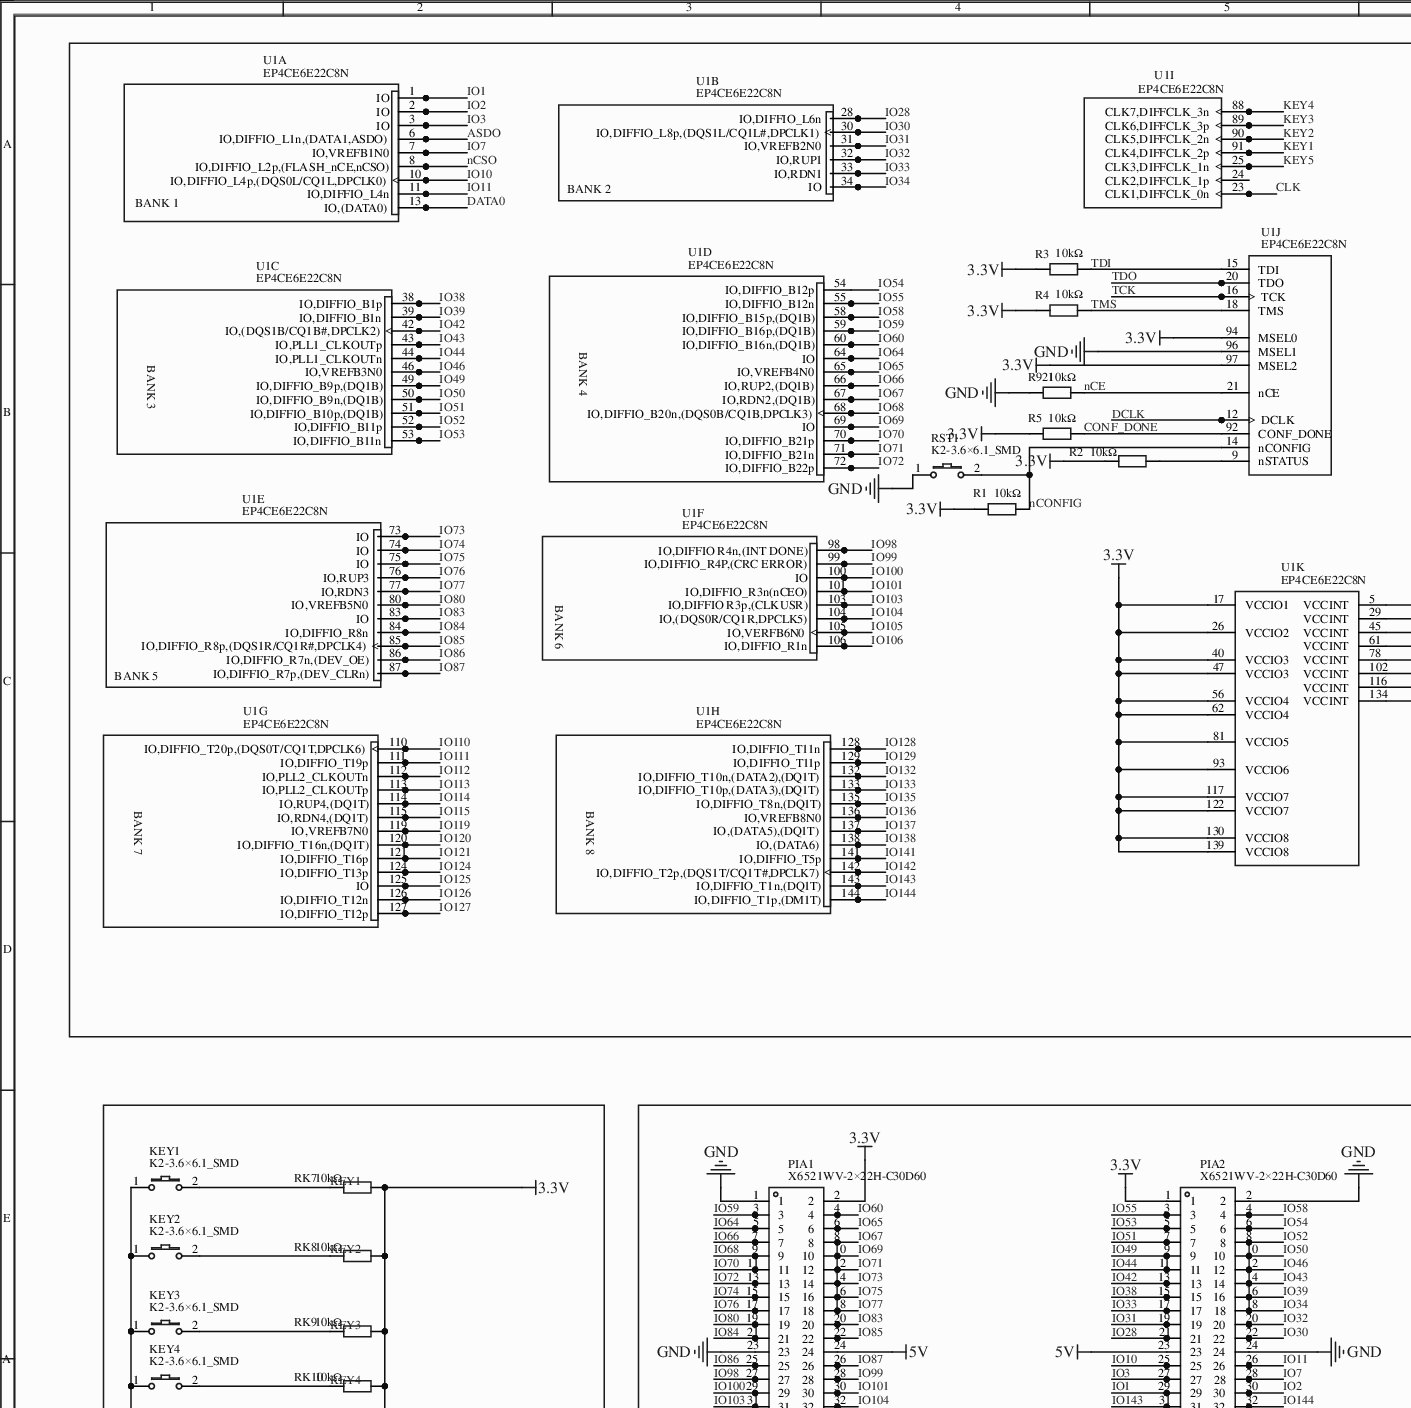
[diagram p0: MISC51540-3.schdoc, top left]
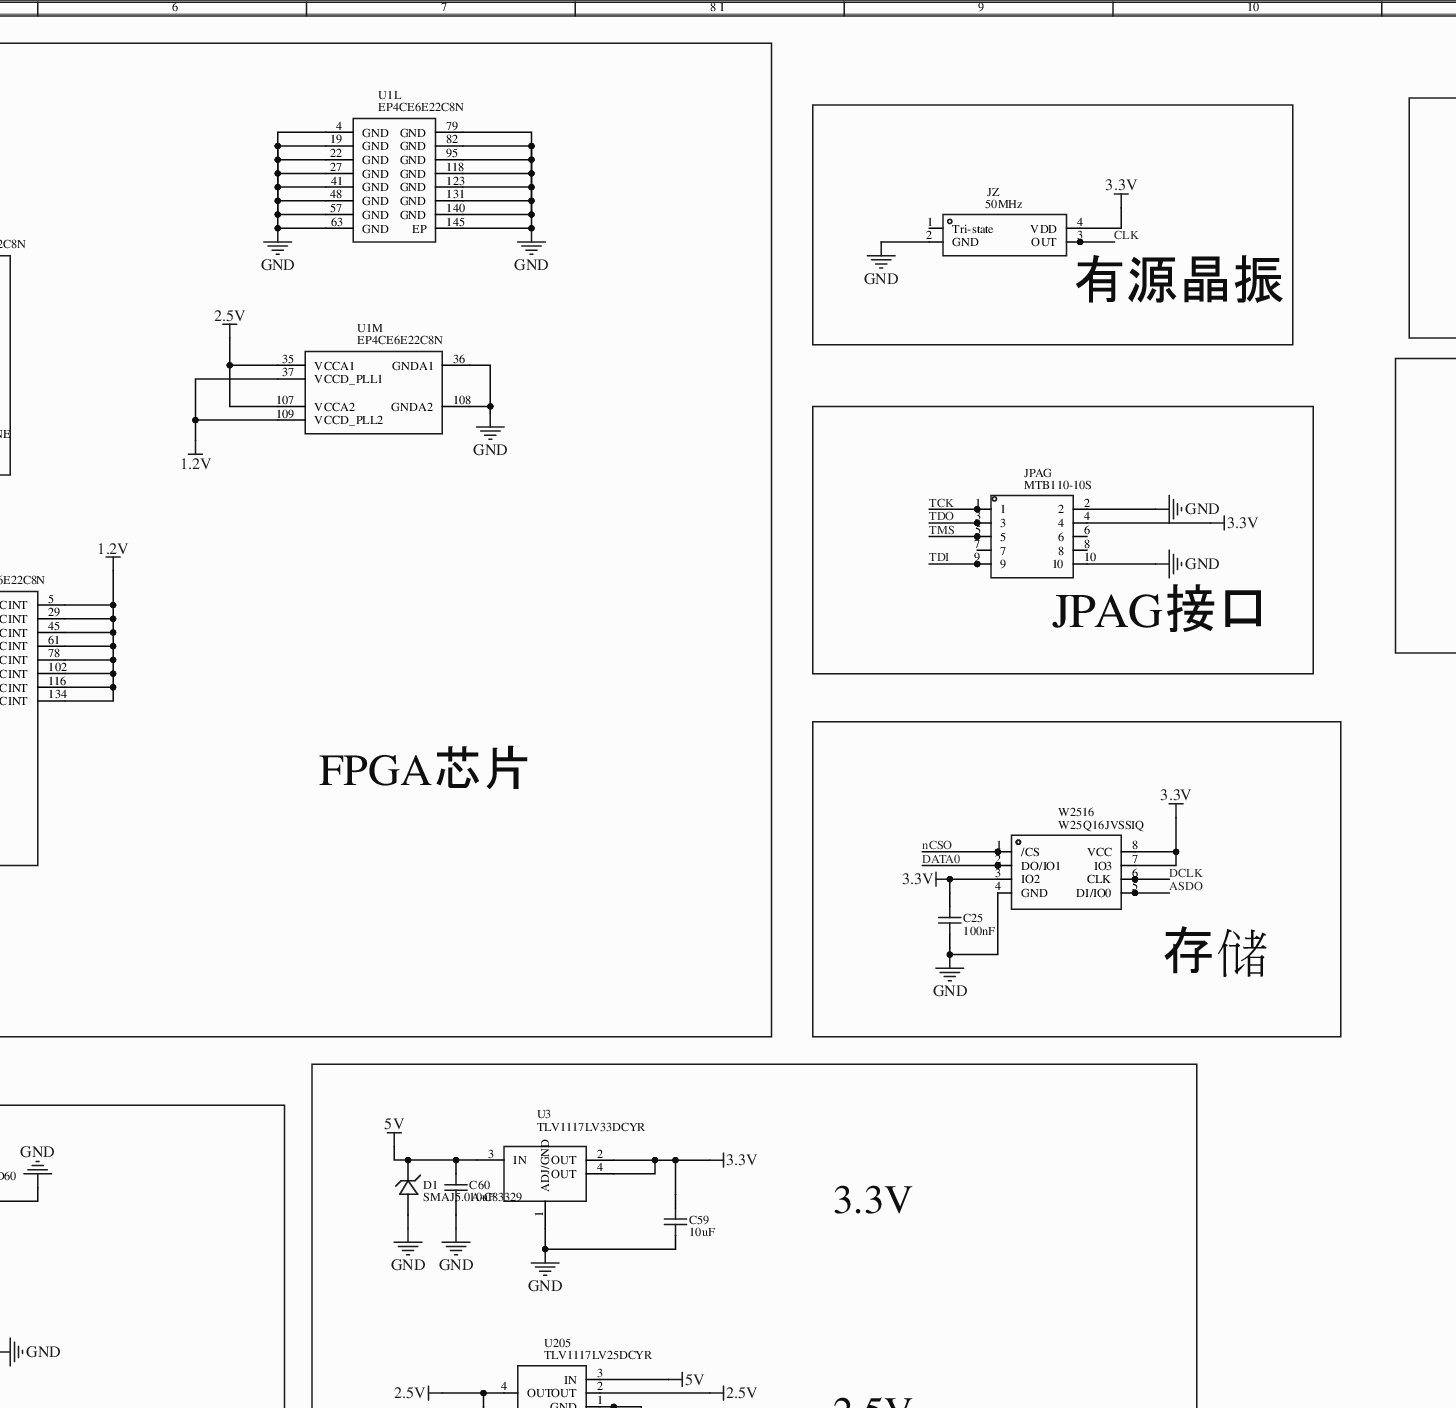
[diagram p1: MISC51540-3.schdoc, top middle]
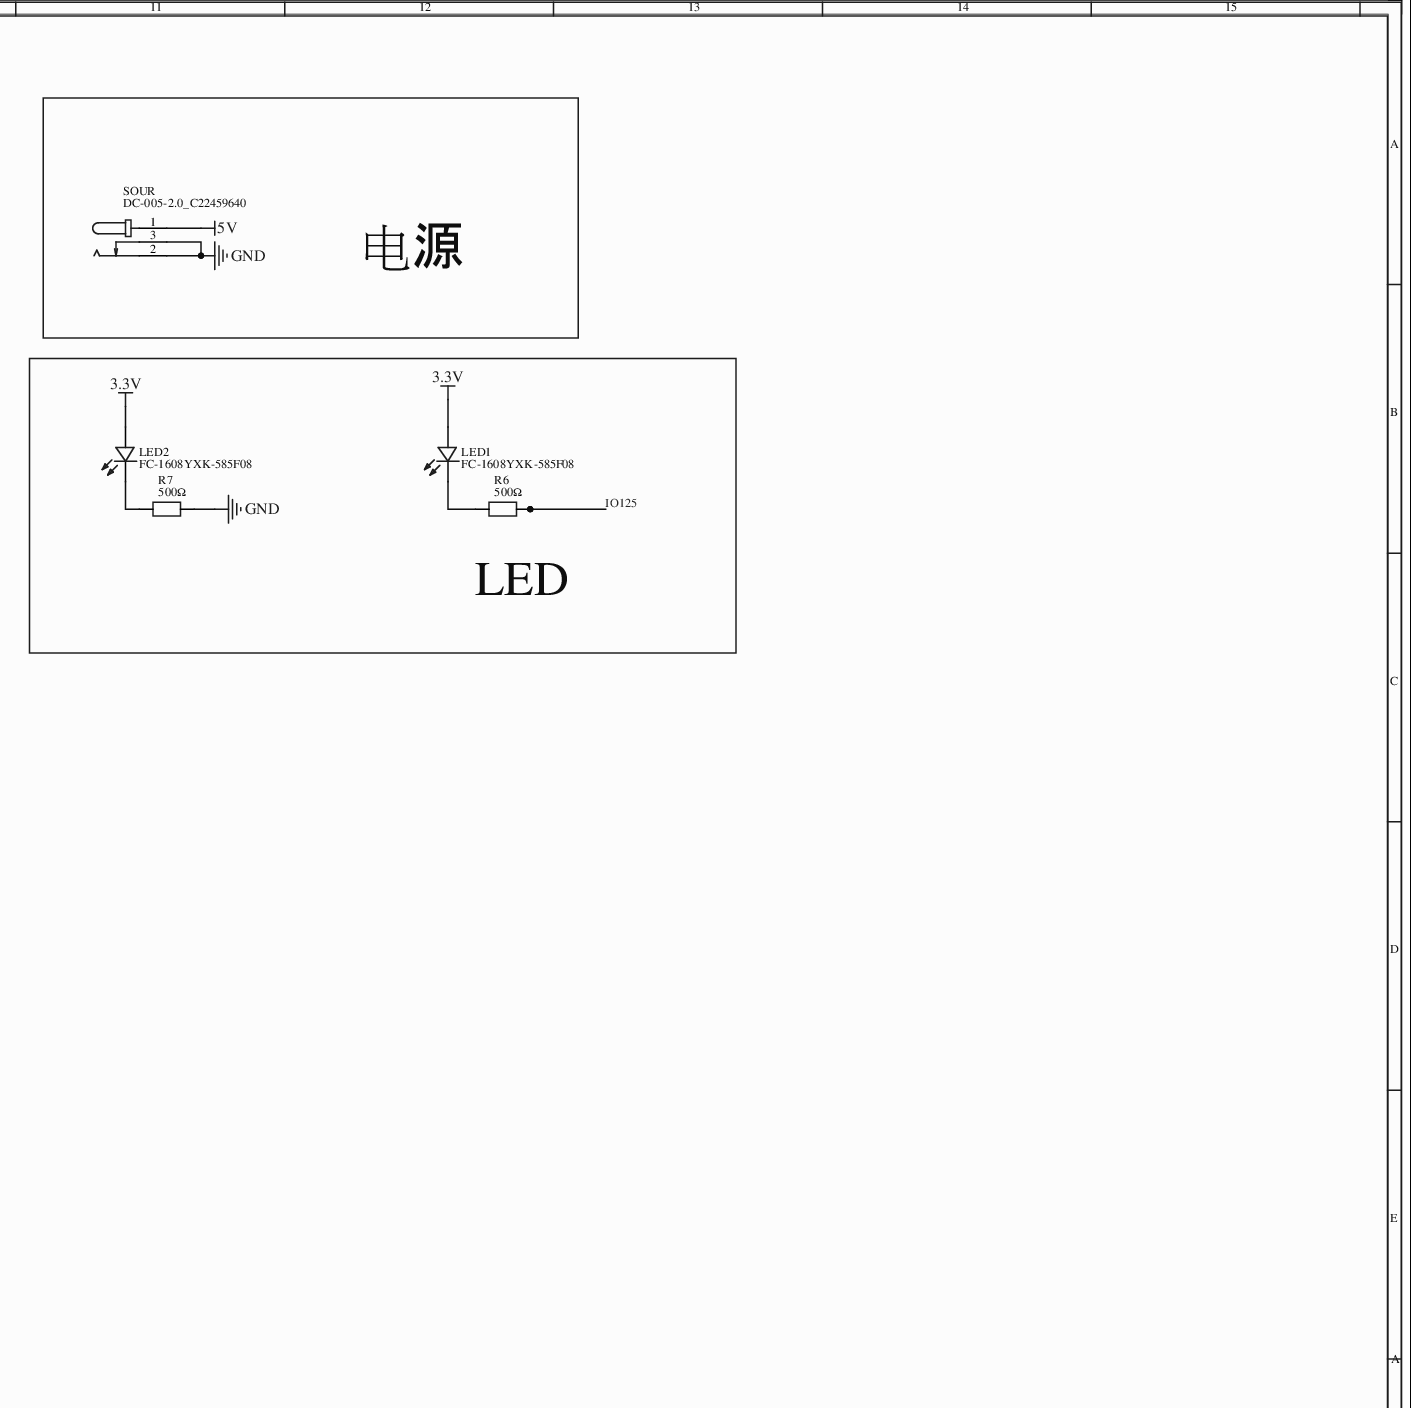
[diagram p2: MISC51540-3.schdoc, top right]
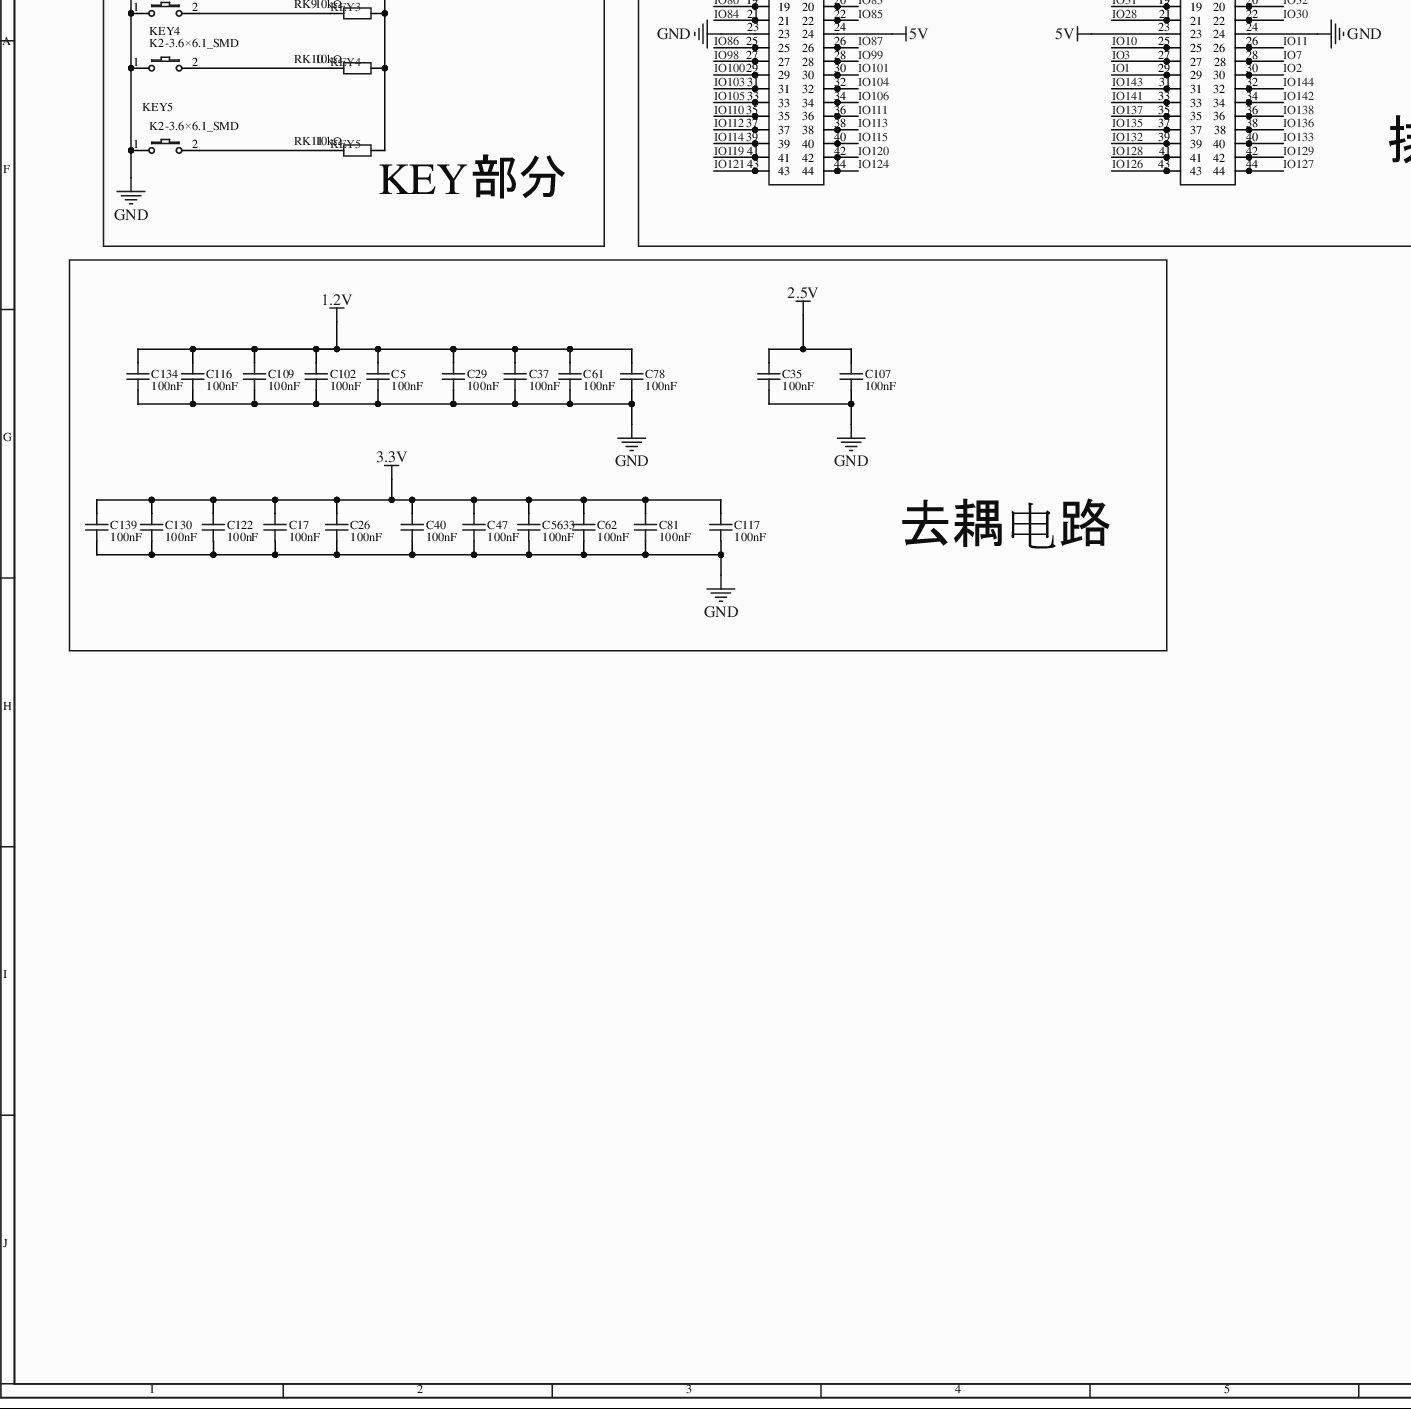
[diagram p3: MISC51540-3.schdoc, bottom left]
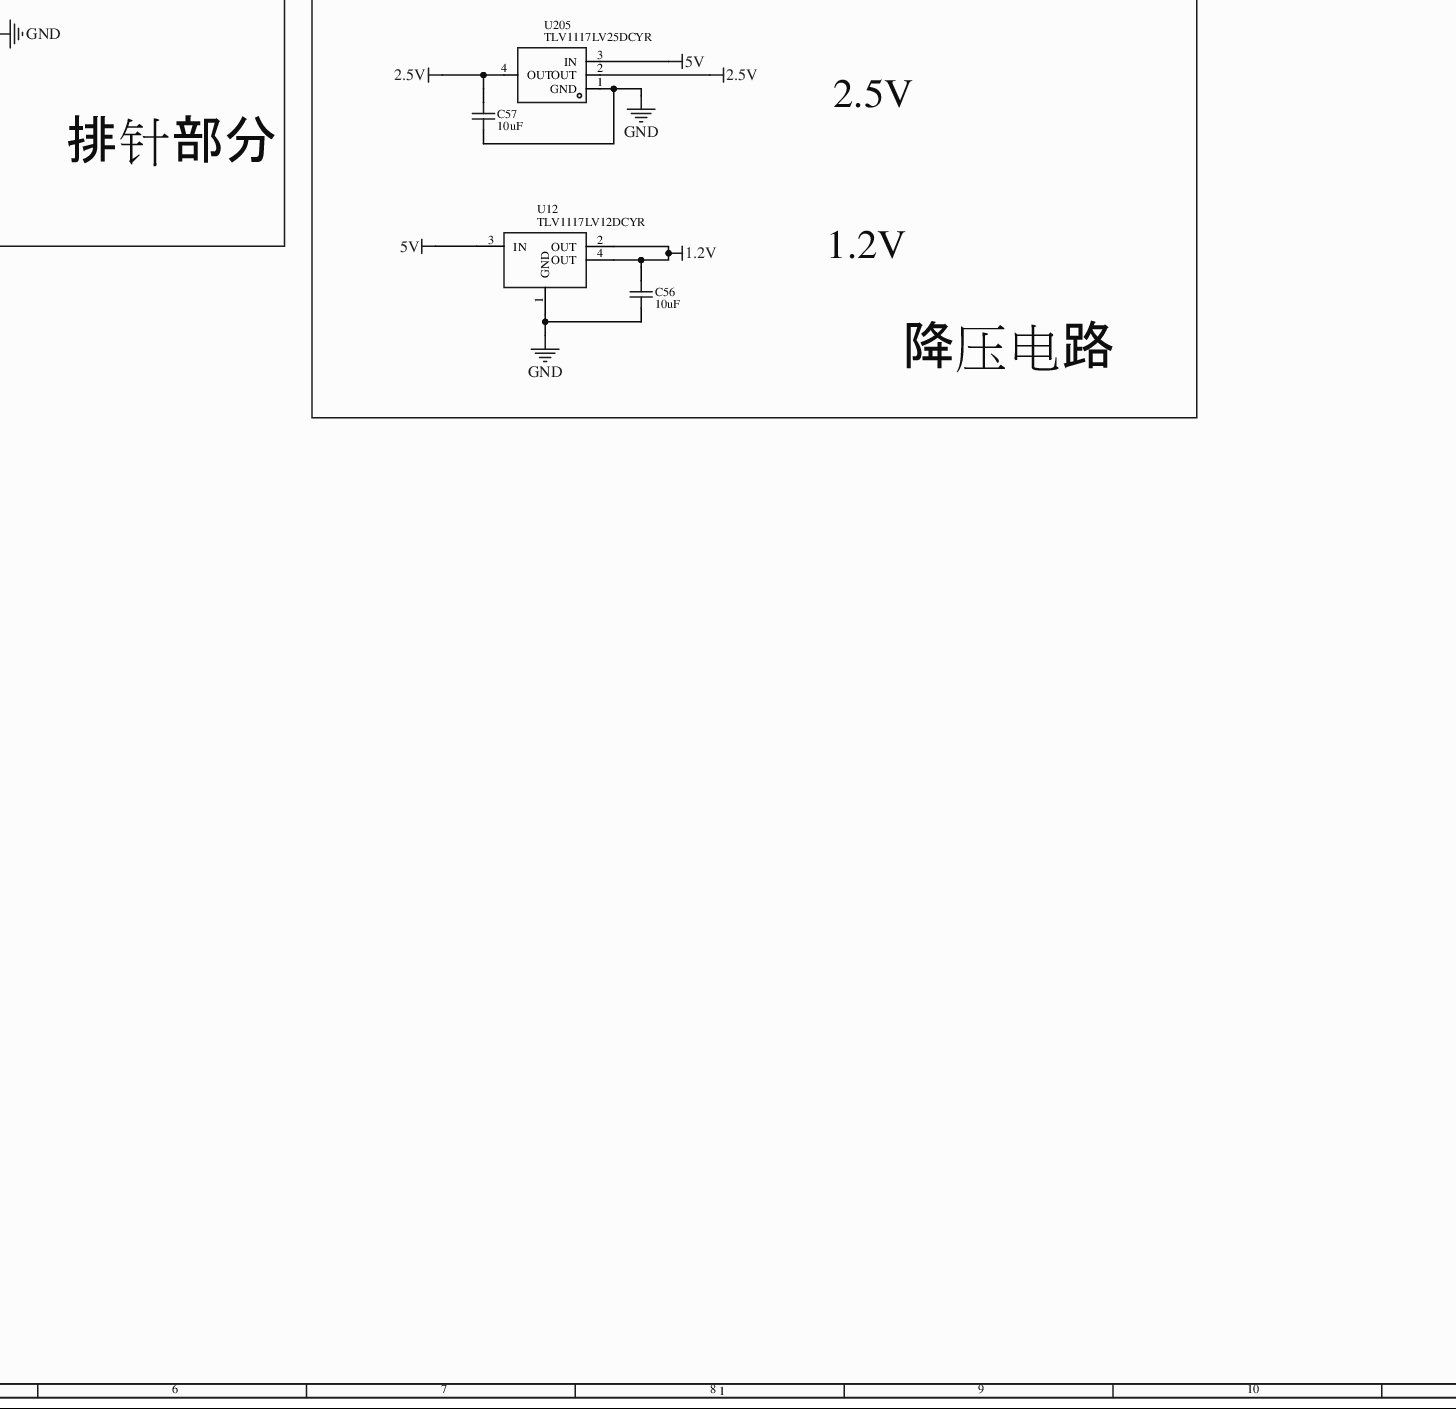
[diagram p4: MISC51540-3.schdoc, bottom middle]
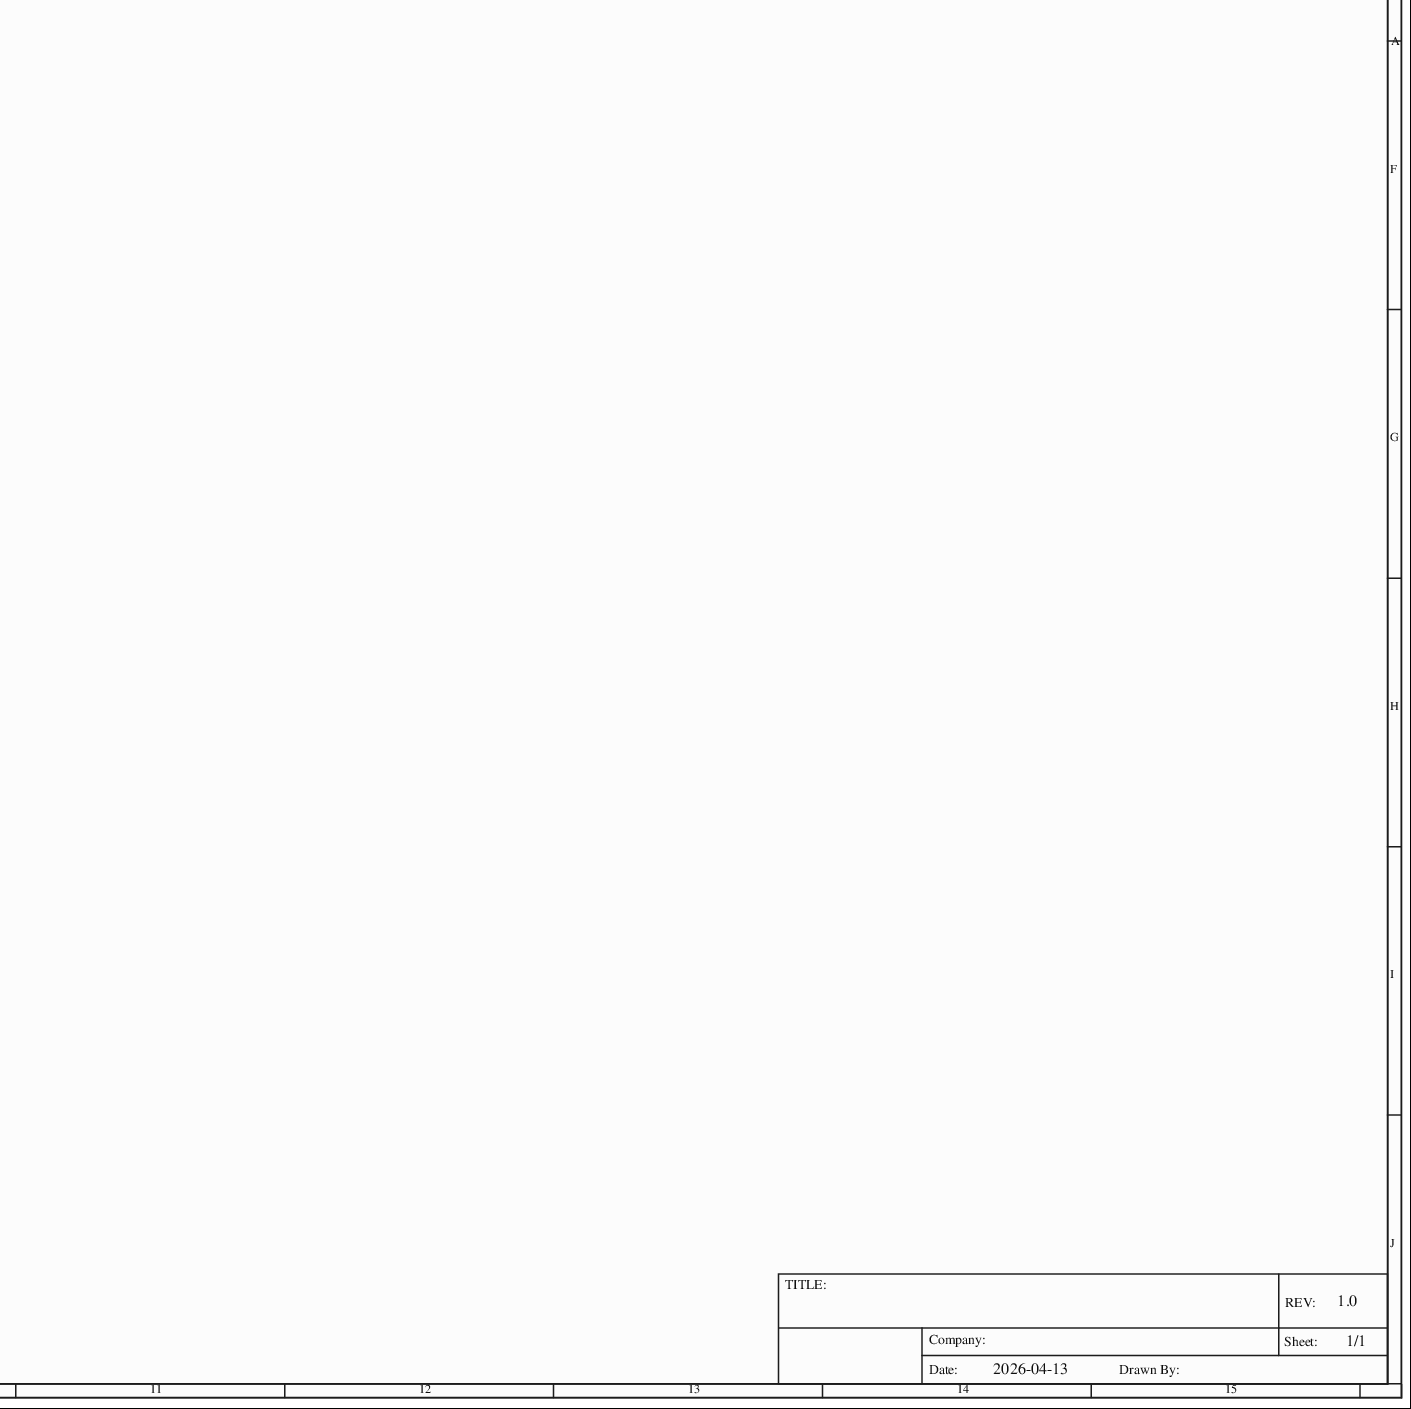
[diagram p5: MISC51540-3.schdoc, bottom right]
# Altium project MISC51540-2.PrjPcb (part 1 of 2)
1 sheet, 59 parts. Net scope: global (net labels, ports and power ports of the same name join across sheets).
Board file: MISC51540.pcbdoc

## Sheet MISC51540-3.schdoc
size 757 x 503 mm; Name: MISC51540; @Project Name: MISC51540; REV: 1.0; Date: 2026-04-13; Sheet: 1/1; Manufacturer Part: ?

### Parts
C5  100nF  [C0603]
C17  100nF  [C0603]
C25  100nF  [C0603]
C26  100nF  [C0603]
C29  100nF  [C0603]
C35  100nF  [C0603]
C37  100nF  [C0603]
C40  100nF  [C0603]
C47  100nF  [C0603]
C56  10uF  [C0603]
C57  10uF  [C0603]
C59  10uF  [C0603]
C60  10uF  [C0603]
C61  100nF  [C0603]
C62  100nF  [C0603]
C78  100nF  [C0603]
C81  100nF  [C0603]
C102  100nF  [C0603]
C107  100nF  [C0603]
C109  100nF  [C0603]
C116  100nF  [C0603]
C117  100nF  [C0603]
C122  100nF  [C0603]
C130  100nF  [C0603]
C134  100nF  [C0603]
C139  100nF  [C0603]
C5633  100nF  [C0603]
D1  SMAJ5.0A-C83329  [SMA_L4.3-W2.6-LS5.2-RD]
JPAG  MTB110-10S  [IDC-TH_MTB110-10S]
JZ  50MHz  [OSC-SMD_4P-L5.0-W3.2-BL_7CZ-XXXXX]
KEY1  K2-3.6×6.1_SMD  [KEY-SMD_2P-L6.2-W3.6-LS8.0]
KEY2  K2-3.6×6.1_SMD  [KEY-SMD_2P-L6.2-W3.6-LS8.0]
KEY3  K2-3.6×6.1_SMD  [KEY-SMD_2P-L6.2-W3.6-LS8.0]
KEY4  K2-3.6×6.1_SMD  [KEY-SMD_2P-L6.2-W3.6-LS8.0]
KEY5  K2-3.6×6.1_SMD  [KEY-SMD_2P-L6.2-W3.6-LS8.0]
LED1  FC-1608YXK-585F08  [LED0603-RD]
LED2  FC-1608YXK-585F08  [LED0603-RD]
PIA1  X6521WV-2×22H-C30D60  [HDR-TH_44P-2.54-V-M-R2-C22-S2.54]
PIA2  X6521WV-2×22H-C30D60  [HDR-TH_44P-2.54-V-M-R2-C22-S2.54]
R1  10kΩ  [R0402]
R2  10kΩ  [R0402]
R3  10kΩ  [R0402]
R4  10kΩ  [R0402]
R5  10kΩ  [R0402]
R6  500Ω  [R0805]
R7  500Ω  [R0805]
R921  10kΩ  [R0402]
RK7  10kΩ  [R0402]
RK8  10kΩ  [R0402]
RK9  10kΩ  [R0402]
RK10  10kΩ  [R0402]
RK11  10kΩ  [R0402]
RST1  K2-3.6×6.1_SMD  [KEY-SMD_2P-L6.2-W3.6-LS8.0]
SOUR  DC-005-2.0_C22459640  [DC-IN-TH_DC-005-2.0_C22459640]
U1  EP4CE6E22C8N  [PQFP-144_L20.0-W20.0-P0.50-LS22.0-BL-EP]  (parts A,B,C,D,E,F,G,H,I,J,K,L,M of 13)
U3  TLV1117LV33DCYR  [SOT-223_L6.7-W3.5-P2.30-BR]
U12  TLV1117LV12DCYR  [SOT-223-4_L6.5-W3.5-P2.30-LS7.0-BR]
U205  TLV1117LV25DCYR  [SOT-223-3_L6.5-W3.4-P2.30-LS7.0-BR]
W2516  W25Q16JVSSIQ  [SOIC-8_L5.3-W5.3-P1.27-LS8.0-BL]

### Blocks framed on the sheet
FPGA芯片: R1-R5 R921 RST1 U1
有源晶振: JZ
电源: SOUR
LED: LED1 LED2 R6 R7
JPAG接口: JPAG
存储: C25 W2516
降压电路: C56 C57 C59 C60 D1 U3 U12 U205
KEY部分: KEY1-KEY5 RK7-RK11